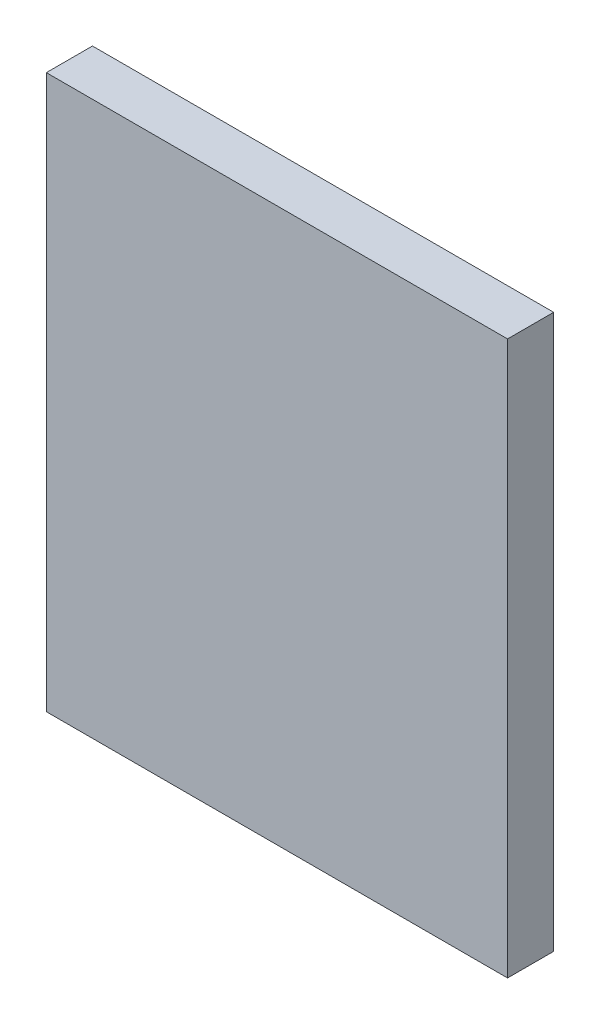
from build123d import *

# Parameters (mm, degrees)
SKETCH_1_W          = 50
SKETCH_1_H          = 150
EXTRUDE_1_DEPTH     = 10
SKETCH_2_W          = 70
SKETCH_2_H          = 30
CUT_EXTRUDE_1_DEPTH = 50
SKETCH_3_W          = 10
SKETCH_3_H          = 100
EXTRUDE_2_DEPTH     = 50
SKETCH_4_W          = 100
SKETCH_4_H          = 10
EXTRUDE_3_DEPTH     = 20


with BuildPart() as part:
    # 草图1 → 凸台-拉伸1 (new body)
    with BuildSketch(Plane.XY):
        with Locations((25, 75)):
            Rectangle(SKETCH_1_W, SKETCH_1_H)
    extrude(amount=EXTRUDE_1_DEPTH)

    # 草图2 → 切除-拉伸1 (cut)
    with BuildSketch(Plane(origin=(0, 150, 0), x_dir=(1, 0, 0), z_dir=(0, 1, 0))):
        with Locations((25, -5)):
            Rectangle(SKETCH_2_W, SKETCH_2_H)
    extrude(amount=-CUT_EXTRUDE_1_DEPTH, mode=Mode.SUBTRACT)

    # 草图3 → 凸台-拉伸2 (add)
    with BuildSketch(Plane.ZY):
        with Locations((5, 50)):
            Rectangle(SKETCH_3_W, SKETCH_3_H)
    extrude(amount=EXTRUDE_2_DEPTH)

    # 草图4 → 凸台-拉伸3 (add)
    with BuildSketch(Plane.XZ):
        with Locations((0, 5)):
            Rectangle(SKETCH_4_W, SKETCH_4_H)
    extrude(amount=EXTRUDE_3_DEPTH)


solid = part.part
